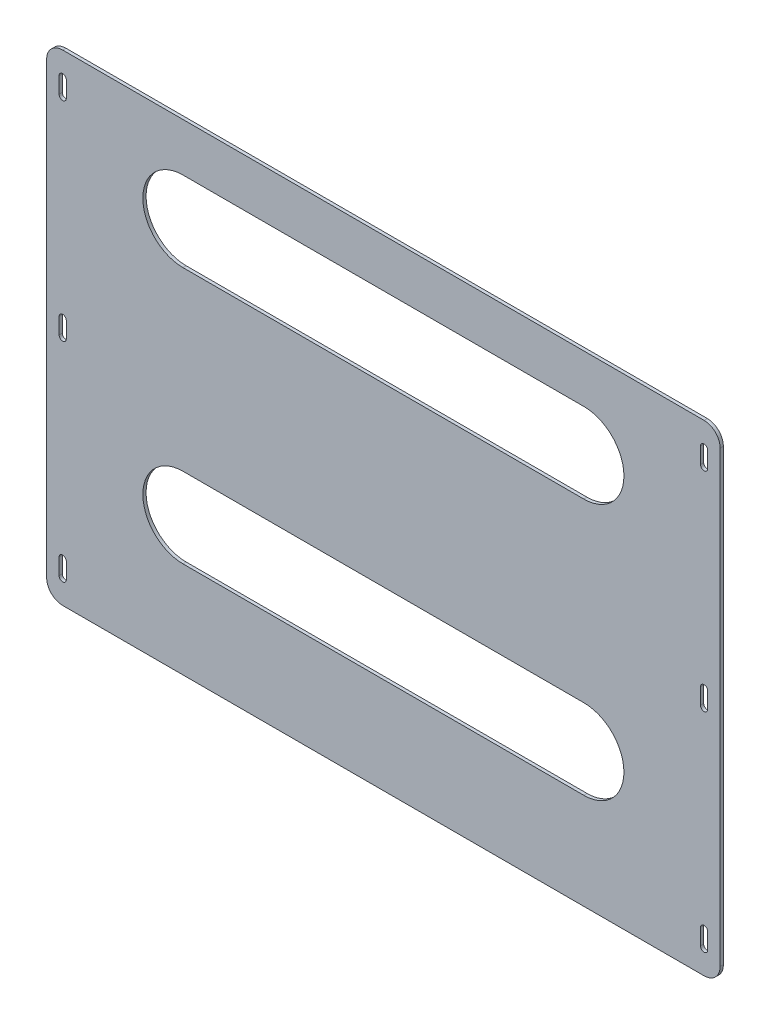
SolidWorks part; units mm, degrees
material "Q235A"
ref_plane "前视基准面" through (0, 0, 0) normal (0, 0, 1) x (1, 0, 0)
ref_plane "上视基准面" through (0, 0, 0) normal (0, 1, 0) x (1, 0, 0)
ref_plane "右视基准面" through (0, 0, 0) normal (1, 0, 0) x (0, 0, -1)
sketch "草图1" plane through (0, 0, 0) normal (0, 0, 1) x (1, 0, 0)
  line L1 (-210, 150) -> (210, 150)
  line L2 (-210, 150) -> (-210, -150)
  line L3 (-210, -150) -> (210, -150)
  line L4 (210, 150) -> (210, -150)
  line L5 (0, -150) -> (0, 150) construction
  line L6 (-210, 0) -> (210, 0) construction
  point P0 (0, 0)
  dimension "D1" = 420
  dimension "D2" = 300
extrude "凸台-拉伸1" add sketch "草图1" along normal blind 2
hole_wizard "M4 螺纹孔的螺纹孔钻头2" positions "草图2" profile "草图3" hole size "M4" standard "GB" end condition through all
sketch "草图2" plane through (0, 0, 2) normal (0, 0, 1) x (1, 0, 0)
  line L2 (-200, -130) -> (200, -130) construction
  line L3 (-200, -130) -> (-200, 0) construction
  line L4 (-200, 0) -> (200, 0) construction
  line L5 (200, -130) -> (200, 0) construction
  line L6 (0, 0) -> (0, -130) construction
  line L7 (-200, -65) -> (200, -65) construction
  line L8 (-210, -150) -> (210, -150) construction
  point P6 (200, 0)
  point P85 (-200, -130)
  point P86 (-200, 0)
  point P87 (200, -130)
  dimension "D1" = 400
  dimension "D3" = 20
sketch "草图3" plane through (200, 0, 2) normal (1, 0, 0) x (0, -1, 0)
  line L0 (0, 0) -> (0, 2)
  line L1 (0, 2) -> (1.65, 2)
  line L2 (1.65, 2) -> (1.65, 0)
  line L5 (1.65, 0) -> (0, 0)
  line L11 (0, -6.35) -> (0, 107.95) construction
  dimension "通孔孔直径" = 3.3
  dimension "通孔孔深度" = 2
sketch "草图4" plane through (0, 0, 2) normal (0, 0, 1) x (1, 0, 0)
  line L5 (-200, -130) -> (200, -130) construction
  line L6 (-200, -130) -> (-200, 0) construction
  line L7 (-200, 0) -> (200, 0) construction
  line L8 (200, -130) -> (200, 0) construction
  line L9 (0, 0) -> (0, -130) construction
  line L10 (-200, -65) -> (200, -65) construction
  line L13 (200, -135) -> (200, -125) construction
  line L14 (197.75, -135) -> (197.75, -125)
  line L15 (202.25, -135) -> (202.25, -125)
  line L16 (-200, -130) -> (-200, 0) construction
  line L17 (-200, -135) -> (-200, -125) construction
  line L18 (-197.75, -135) -> (-197.75, -125)
  line L19 (-202.25, -135) -> (-202.25, -125)
  line L23 (-210, 0) -> (210, 0) construction
  line L24 (-210, 150) -> (-210, -150) construction
  line L25 (210, -150) -> (210, 150) construction
  line L26 (200, -5) -> (200, 5) construction
  line L27 (202.25, -5) -> (202.25, 5)
  line L28 (197.75, -5) -> (197.75, 5)
  line L29 (200, 135) -> (200, 125) construction
  line L30 (197.75, 135) -> (197.75, 125)
  line L31 (202.25, 135) -> (202.25, 125)
  line L32 (-200, 135) -> (-200, 125) construction
  line L33 (-197.75, 135) -> (-197.75, 125)
  line L34 (-202.25, 135) -> (-202.25, 125)
  line L35 (-200, -5) -> (-200, 5) construction
  line L36 (-202.25, -5) -> (-202.25, 5)
  line L37 (-197.75, -5) -> (-197.75, 5)
  line L38 (-200, 130) -> (-200, 0) construction
  line L39 (-200, 65) -> (200, 65) construction
  line L40 (0, 0) -> (0, 130) construction
  line L41 (200, 130) -> (200, 0) construction
  line L42 (-200, 0) -> (200, 0) construction
  line L43 (-200, 130) -> (-200, 0) construction
  line L44 (-200, 130) -> (200, 130) construction
  circle A0 centre (-200, -130) radius 1.65 construction
  arc A3 (197.75, -135) -> (202.25, -135) centre (200, -135) ccw
  arc A4 (202.25, -125) -> (197.75, -125) centre (200, -125) ccw
  arc A5 (-197.75, -135) -> (-202.25, -135) centre (-200, -135) cw
  arc A6 (-202.25, -125) -> (-197.75, -125) centre (-200, -125) cw
  arc A9 (202.25, -5) -> (197.75, -5) centre (200, -5) cw
  arc A10 (197.75, 5) -> (202.25, 5) centre (200, 5) cw
  arc A11 (197.75, 135) -> (202.25, 135) centre (200, 135) cw
  arc A12 (202.25, 125) -> (197.75, 125) centre (200, 125) cw
  arc A13 (-197.75, 135) -> (-202.25, 135) centre (-200, 135) ccw
  arc A14 (-202.25, 125) -> (-197.75, 125) centre (-200, 125) ccw
  arc A15 (-202.25, -5) -> (-197.75, -5) centre (-200, -5) ccw
  arc A16 (-197.75, 5) -> (-202.25, 5) centre (-200, 5) ccw
  point P0 (0, 0)
  point P12 (200, -130)
  point P20 (-200, -130)
  point P42 (200, 0)
  point P49 (200, 130)
  point P56 (-200, 130)
  point P63 (-200, 0)
  dimension "D1" = 10
  dimension "D3" = 4.5
extrude "切除-拉伸1" cut sketch "草图4" against normal blind 10
fillet "圆角1" radius 10 4 edges at (-210, -150, 1) (-210, 150, 1) (210, -150, 1) (210, 150, 1)
sketch "草图5" plane through (0, 0, 2) normal (0, 0, 1) x (1, 0, 0)
  line L0 (0, 150) -> (0, -150) construction
  line L1 (200, 150) -> (-200, 150) construction
  line L2 (-200, -150) -> (200, -150) construction
  line L3 (0, -65) -> (109.8805, -65) construction
  line L4 (109.8805, -65) -> (103.6586, -63.0872) construction
  line L5 (-125, -65) -> (125, -65) construction
  line L6 (-125, -40) -> (125, -40)
  line L7 (-125, -90) -> (125, -90)
  line L8 (125, 95) -> (-125, 95) construction
  line L9 (125, 70) -> (-125, 70)
  line L10 (125, 120) -> (-125, 120)
  arc A0 (-125, -40) -> (-125, -90) centre (-125, -65) ccw
  arc A1 (125, -90) -> (125, -40) centre (125, -65) ccw
  arc A2 (125, 70) -> (125, 120) centre (125, 95) ccw
  arc A3 (-125, 120) -> (-125, 70) centre (-125, 95) ccw
  point P11 (0, -65)
  point P18 (0, 95)
  dimension "D1" = 50
  dimension "D2" = 250
  dimension "D3" = 60
  dimension "D4" = 30
extrude "切除-拉伸2" cut sketch "草图5" against normal blind 10
mirror "镜向1" [suppressed] about plane through (0, 0, 0) normal (0, 1, 0)
ref_plane "基准面4" through (0, -20, 0) normal (0, 1, 0) x (1, 0, 0)
